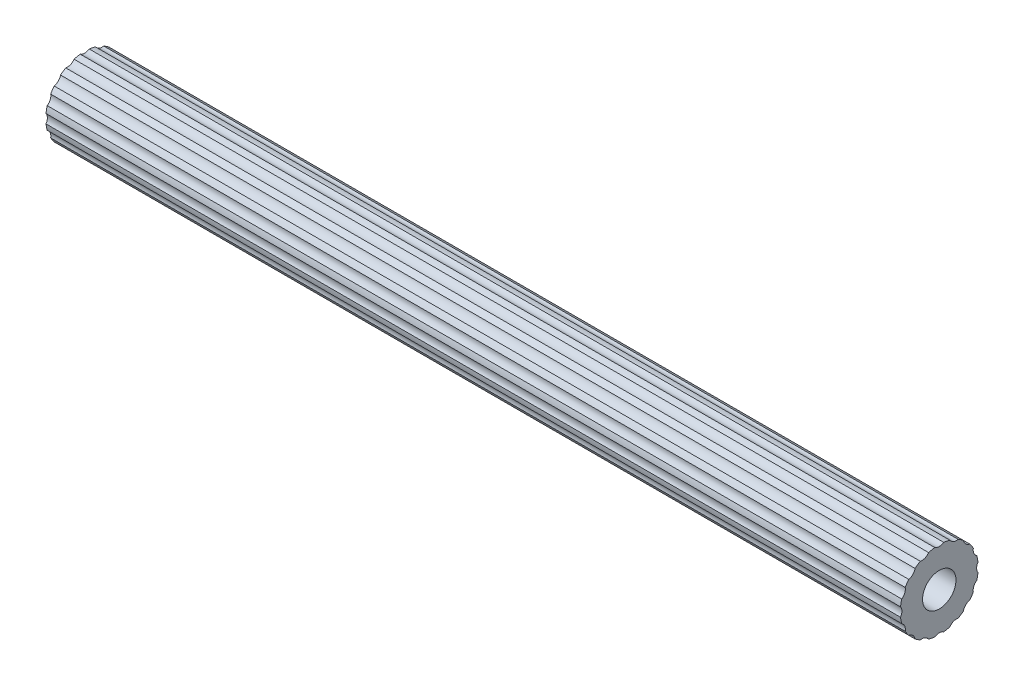
SolidWorks part; units mm, degrees
ref_plane "Front Plane" through (0, 0, 0) normal (0, 0, 1) x (1, 0, 0)
ref_plane "Top Plane" through (0, 0, 0) normal (0, 1, 0) x (1, 0, 0)
ref_plane "Right Plane" through (0, 0, 0) normal (1, 0, 0) x (0, 0, -1)
sketch "Sketch1" plane through (0, 0, 0) normal (1, 0, 0) x (0, 0, -1)
  circle A0 centre (0, 0) radius 35
  circle A1 centre (0, 0) radius 15
extrude "Boss-Extrude2" add sketch "Sketch1" along normal blind 767
sketch "Sketch2" plane through (0, 0, 0) normal (-1, 0, 0) x (0, 0, 1)
  circle A0 centre (0, 40.7409) radius 7.2035
extrude "Cut-Extrude1" cut sketch "Sketch2" against normal blind 767
pattern_circular "Pattern(Circular)1" count 16 over 360 about axis through (0, 0, 0) along (1, 0, 0) of "Cut-Extrude1"
